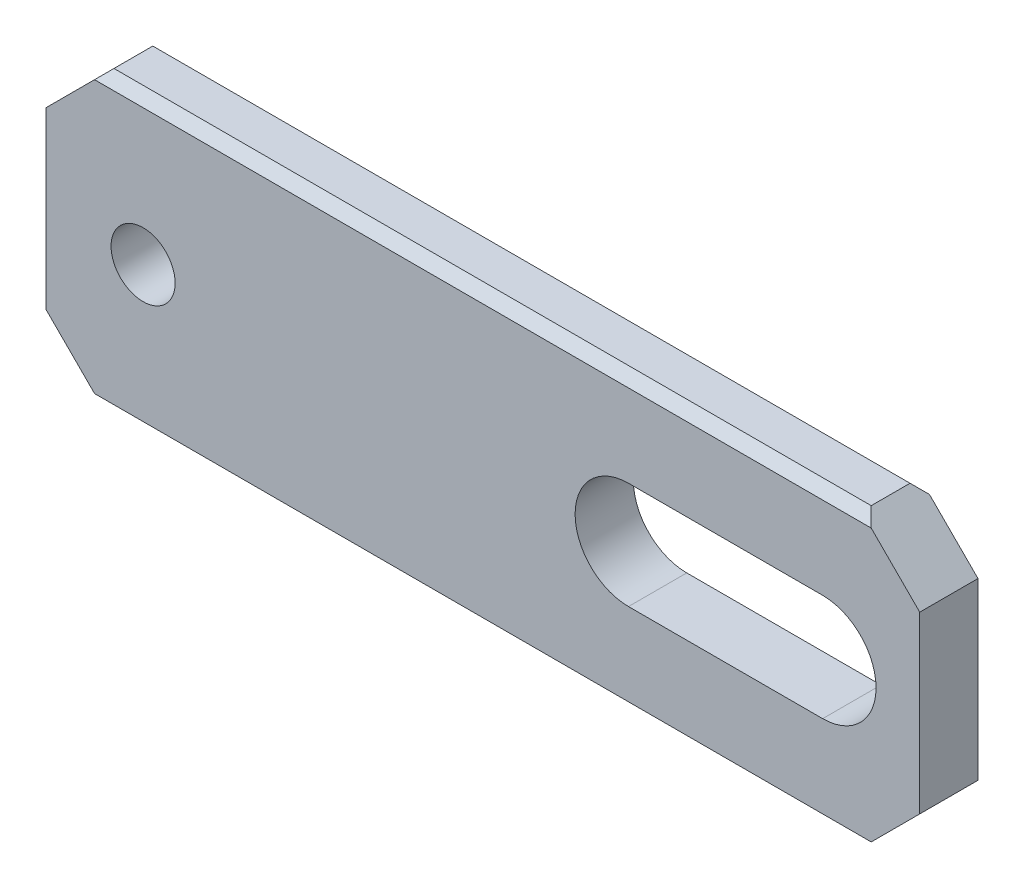
SolidWorks part; units mm, degrees
material "SUS304"
ref_plane "Front Plane" through (0, 0, 0) normal (0, 0, 1) x (1, 0, 0)
ref_plane "Top Plane" through (0, 0, 0) normal (0, 1, 0) x (1, 0, 0)
ref_plane "Right Plane" through (0, 0, 0) normal (1, 0, 0) x (0, 0, -1)
sketch "Sketch1" plane through (0, 0, 0) normal (0, 0, 1) x (1, 0, 0)
  line L1 (-22.5, -7.5) -> (22.5, -7.5)
  line L2 (-22.5, -7.5) -> (-22.5, 7.5)
  line L3 (-22.5, 7.5) -> (22.5, 7.5)
  line L4 (22.5, -7.5) -> (22.5, 7.5)
  line L5 (-22.5, -7.5) -> (22.5, 7.5) construction
  line L6 (-22.5, 7.5) -> (22.5, -7.5) construction
  point P0 (0, 0)
  dimension "D1" = 45
  dimension "D2" = 15
extrude "Boss-Extrude1" add sketch "Sketch1" along normal blind 3
hole_wizard "M4 Tapped Hole1" positions "Sketch3" profile "Sketch2" tap size "M4" standard "GB"
sketch "Sketch3" plane through (0, 0, 3) normal (0, 0, 1) x (1, 0, 0)
  line L0 (-22.5, 7.5) -> (-22.5, -7.5) construction
  point P0 (-17.5, 0)
  dimension "D1" = 5
sketch "Sketch2" plane through (-17.5, 0, 3) normal (1, 0, 0) x (0, -1, 0)
  line L0 (0, 0) -> (0, 11.0914)
  line L1 (0, 11.0914) -> (1.65, 10.1)
  line L2 (1.65, 10.1) -> (1.65, 0)
  line L5 (1.65, 0) -> (0, 0)
  line L10 (0, 11.0914) -> (-1.65, 10.1) construction
  line L11 (0, -6.35) -> (0, 107.95) construction
  dimension "螺纹孔钻头直径" = 3.3
  dimension "螺纹孔钻头深度" = 10.1
  dimension "导头角度" = 118
cosmetic thread "Cosmetic Thread1" parameters "D1"=3, "D2"=4
sketch "Sketch4" plane through (0, 0, 3) normal (0, 0, 1) x (1, 0, 0)
  line L0 (7.5, 0) -> (17.5, 0) construction
  line L1 (7.5, 2.75) -> (17.5, 2.75)
  line L2 (7.5, -2.75) -> (17.5, -2.75)
  line L3 (22.5, -7.5) -> (22.5, 7.5) construction
  arc A0 (7.5, 2.75) -> (7.5, -2.75) centre (7.5, 0) ccw
  arc A1 (17.5, -2.75) -> (17.5, 2.75) centre (17.5, 0) ccw
  point P3 (12.5, 0)
  dimension "D1" = 10
  dimension "D2" = 5.5
  dimension "D3" = 5
extrude "Cut-Extrude1" cut sketch "Sketch4" against normal blind 3
chamfer "Chamfer1" distance 3 angle 45 4 edges at (22.5, -7.5, 1.5) (22.5, 7.5, 1.5) (-22.5, -7.5, 1.5) (-22.5, 7.5, 1.5)
chamfer "Chamfer2" distance 0.5 angle 45 4 edges at (0, 7.5, 3) (0, -7.5, 3) (0, 7.5, 0) (0, -7.5, 0)
